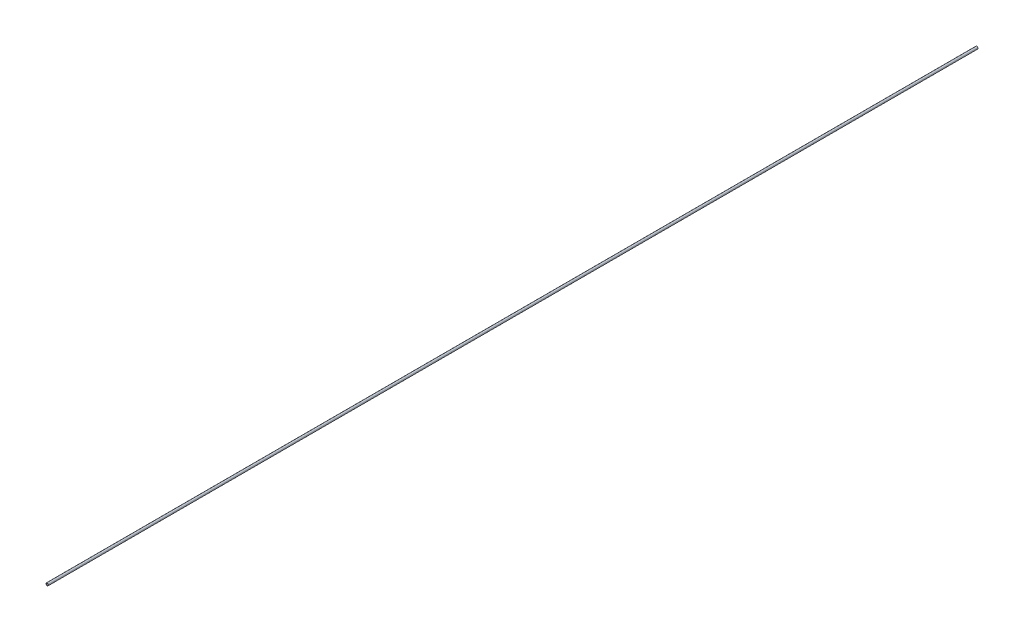
from build123d import *

# Parameters (mm, degrees)
SKETCH1_R           = 9.525
SKETCH1_R_2         = 6.775
BOSS_EXTRUDE1_DEPTH = 3664.5


with BuildPart() as part:
    # Sketch1 → Boss-Extrude1 (new, symmetric)
    with BuildSketch(Plane.XY):
        Circle(SKETCH1_R)
        Circle(SKETCH1_R_2, mode=Mode.SUBTRACT)
    extrude(amount=BOSS_EXTRUDE1_DEPTH, both=True)


solid = part.part
